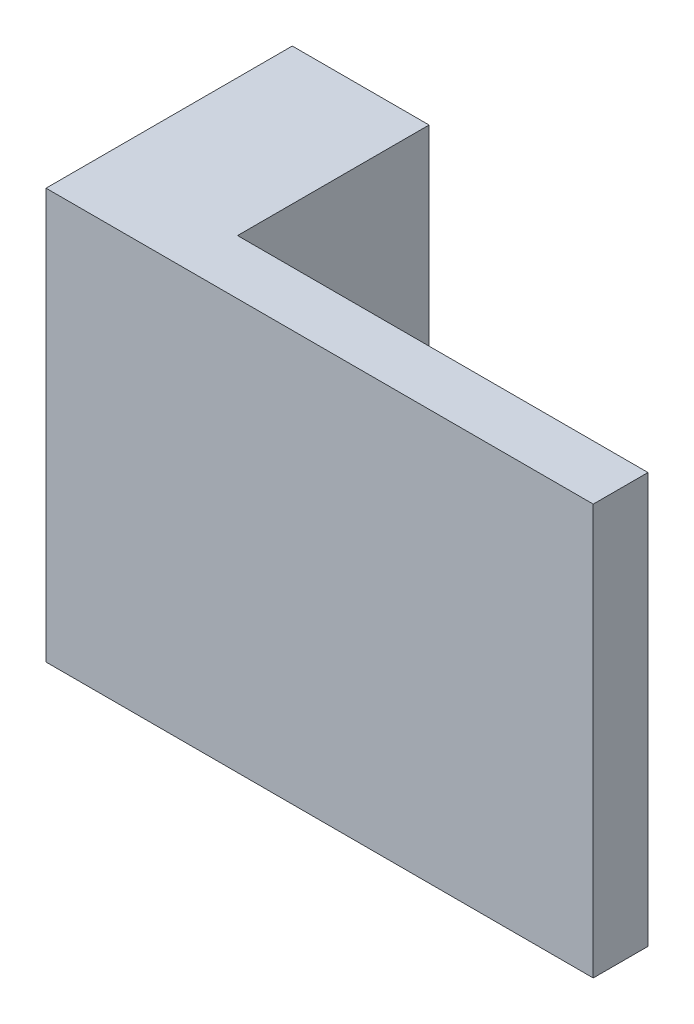
from build123d import *

# Parameters (mm, degrees)
SKETCH1_W           = 5
SKETCH1_H           = 15
BOSS_EXTRUDE1_DEPTH = 7
SKETCH2_W           = 20
SKETCH2_H           = 15
BOSS_EXTRUDE2_DEPTH = 2


with BuildPart() as part:
    # Sketch1 → Boss-Extrude1 (new body)
    with BuildSketch(Plane.XY):
        Rectangle(SKETCH1_W, SKETCH1_H)
    extrude(amount=BOSS_EXTRUDE1_DEPTH)

    # Sketch2 → Boss-Extrude2 (add)
    with BuildSketch(Plane.XY.offset(7)):
        with Locations((7.5, 0)):
            Rectangle(SKETCH2_W, SKETCH2_H)
    extrude(amount=BOSS_EXTRUDE2_DEPTH)


solid = part.part
